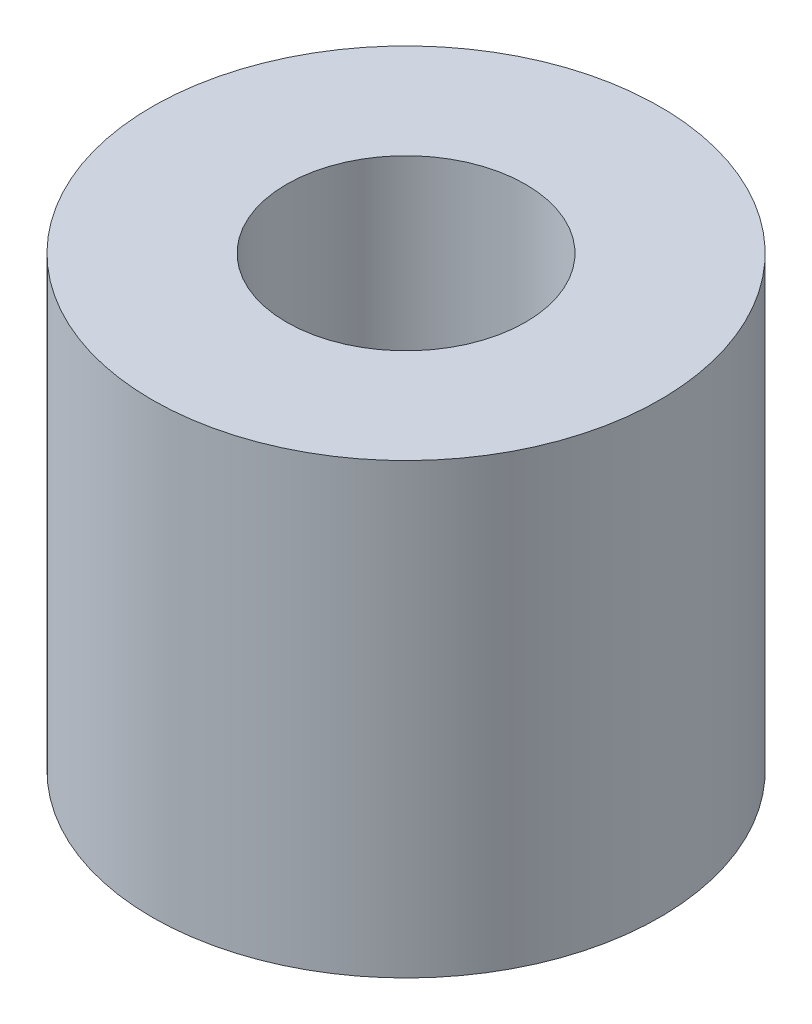
SolidWorks part; units mm, degrees
ref_plane "前视基准面" through (0, 0, 0) normal (0, 0, 1) x (1, 0, 0)
ref_plane "上视基准面" through (0, 0, 0) normal (0, 1, 0) x (1, 0, 0)
ref_plane "右视基准面" through (0, 0, 0) normal (1, 0, 0) x (0, 0, -1)
other "Configuration Table"
sketch "草图1" plane through (0, 0, 0) normal (0, 1, 0) x (1, 0, 0)
  circle A0 centre (0, 0) radius 1.6
  circle A1 centre (0, 0) radius 3.4
  dimension "D1" = 3.2
  dimension "D2" = 6.8
extrude "凸台-拉伸1" add sketch "草图1" along normal blind 6
